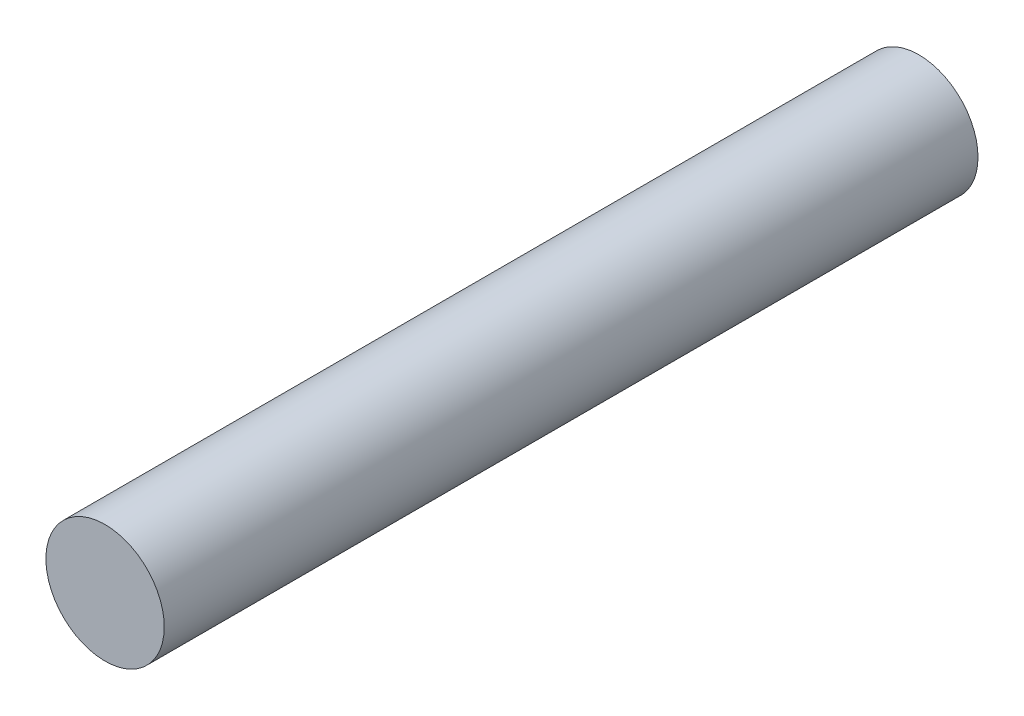
from build123d import *

# Parameters (mm, degrees)
SKETCH_1_R      = 4
EXTRUDE_1_DEPTH = 27.5


with BuildPart() as part:
    # 草图1 → 凸台-拉伸1 (new, symmetric)
    with BuildSketch(Plane.XY):
        Circle(SKETCH_1_R)
    extrude(amount=EXTRUDE_1_DEPTH, both=True)


solid = part.part
